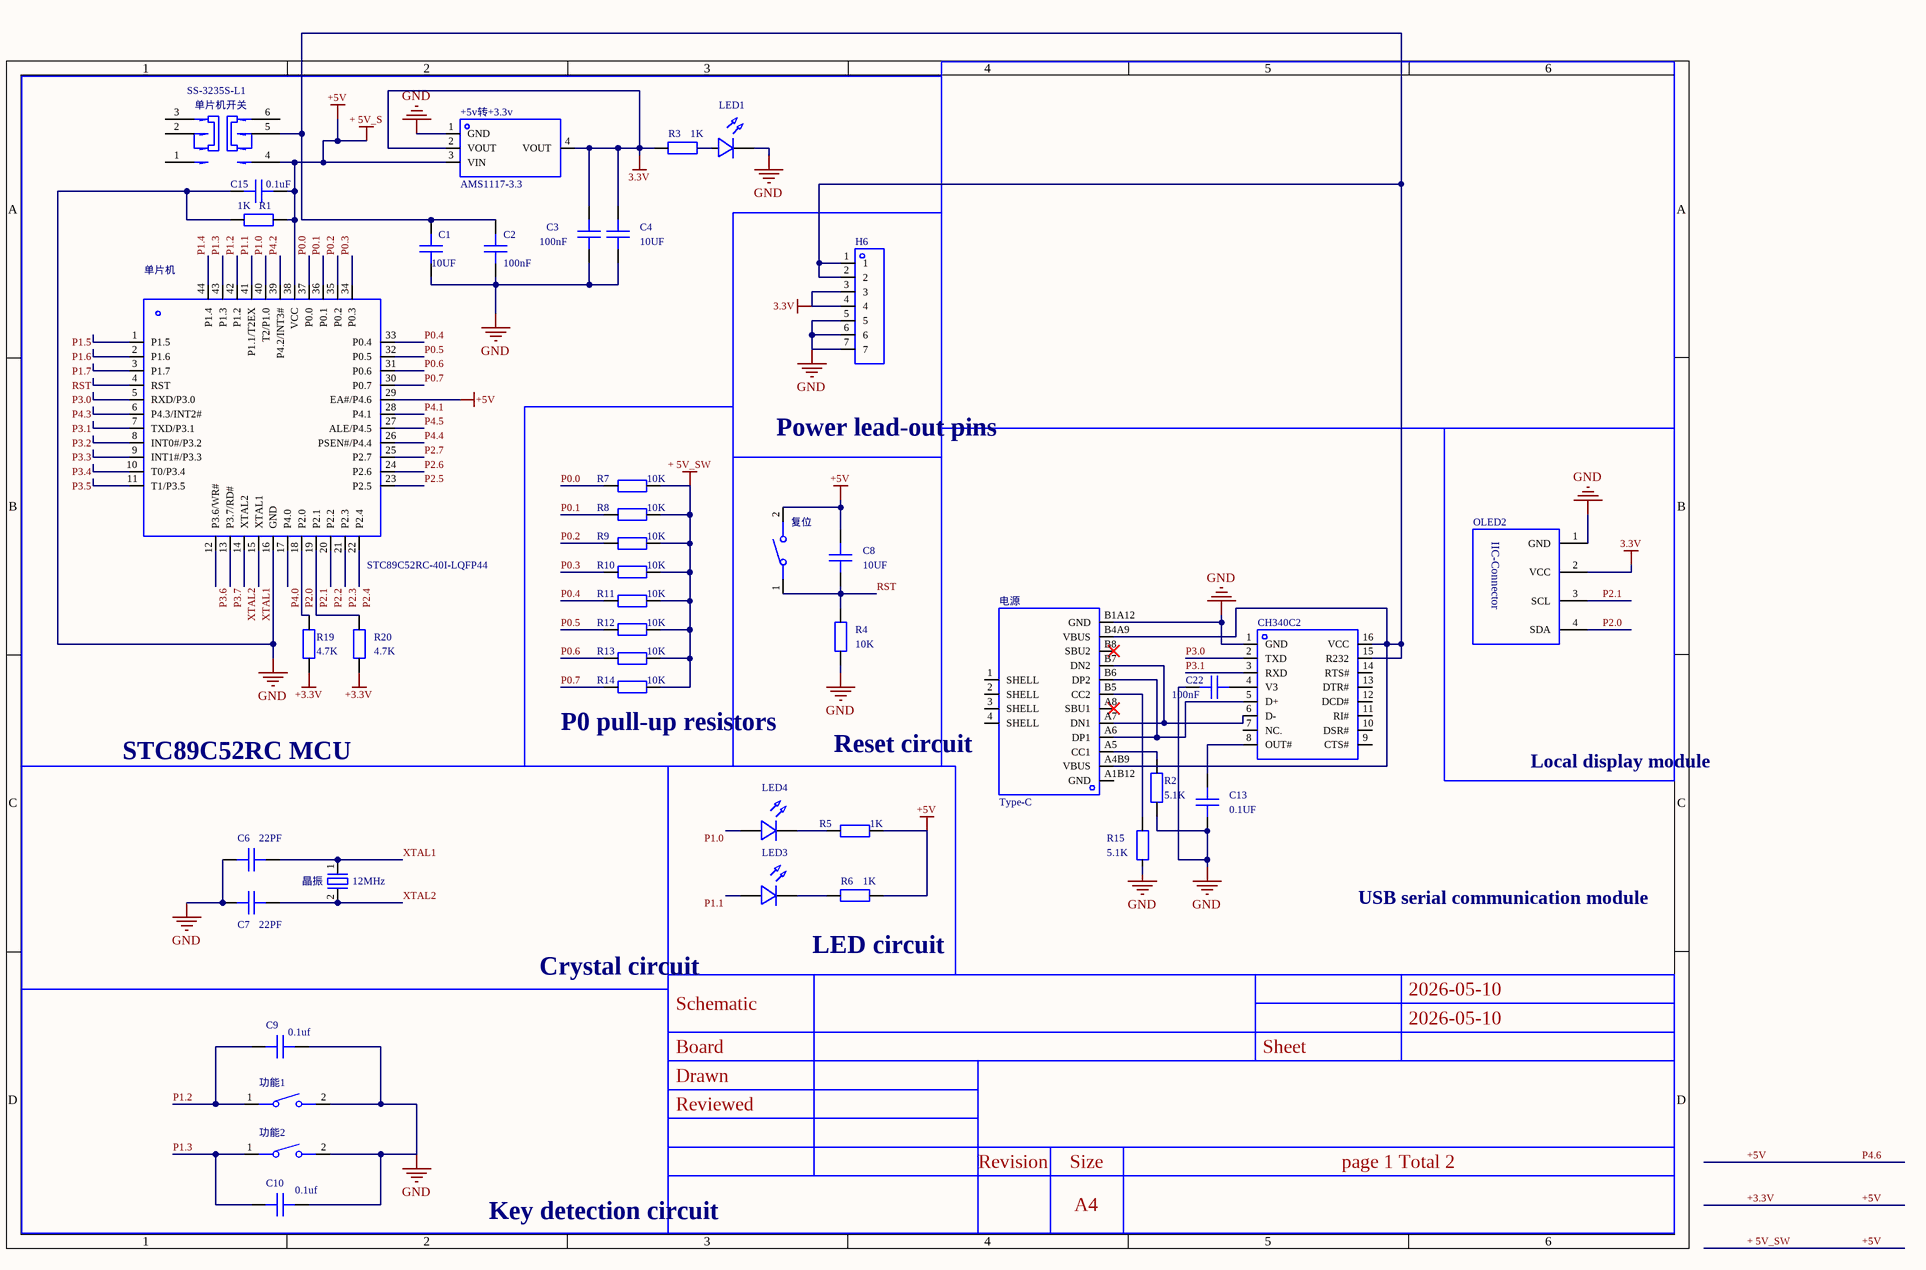
[diagram p0: MISC75115-3.schdoc]
# Altium project MISC75115-2.PrjPcb
2 sheets, 101 parts. Net scope: global (net labels, ports and power ports of the same name join across sheets).
Board file: MISC75115.pcbdoc
Sheets:
  MISC75115-3.schdoc
  MISC75115-4.schdoc

## Sheet MISC75115-3.schdoc
size 297 x 209 mm; Version: V1.0; @Project Name: MISC75115; @Page Count: 2; @Update Date: 2026-05-22; @Create Date: 2026-05-22; @Schematic Name: MISC75115; @Page No: 1; @Board Name: MISC75115; @Create Time: 00:24:12; @Update Time: 02:37:15; Size: A4

### Parts
+5v转+3.3v  AMS1117-3.3  [SOT-223-3_L6.5-W3.4-P2.30-LS7.0-BR]
C1  10UF  [C0805]
C2  100nF  [C0805]
C3  100nF  [C0805]
C4  10UF  [C0805]
C6  22PF  [C0805]
C7  22PF  [C0805]
C8  10UF  [C0805]
C9  0.1uf  [C0805]
C10  0.1uf  [C0805]
C13  0.1UF  [C0805]
C15  0.1uF  [C0805]
C22  100nF  [C0603]
CH340C2  CH340C  [SOP-16_L10.0-W3.9-P1.27-LS6.0-BL]  (value not drawn)
H6  (no value)  [HDR-TH_7P-P2.54-V-M]
LED1  (no value)  [LED_0805]
LED3  (no value)  [LED_0805]
LED4  (no value)  [LED_0805]
OLED2  0.96OLED_4P_MODULE_JX  [0.96OLED_4P]  (value not drawn)
R1  1K  [R0805]
R2  5.1K  [R0603]
R3  1K  [R0805]
R4  10K  [R0805]
R5  1K  [R0805]
R6  1K  [R0805]
R7  10K  [R0805]
R8  10K  [R0805]
R9  10K  [R0805]
R10  10K  [R0805]
R11  10K  [R0805]
R12  10K  [R0805]
R13  10K  [R0805]
R14  10K  [R0805]
R15  5.1K  [R0603]
R19  4.7K  [R0603]
R20  4.7K  [R0603]
功能1  Tact switch 3*4*H  [SW-SMD_L4.0-W2.9-LS5.0]  (value not drawn)
功能2  Tact switch 3*4*H  [SW-SMD_L4.0-W2.9-LS5.0]  (value not drawn)
单片机  STC89C52RC-40I-LQFP44  [LQFP-44_L10.0-W10.0-P0.80-LS12.0-BL]
单片机开关  SS-3235S-L1  [SW-SMD_SS-3235S-LX]
复位  Tact switch 3*4*H  [SW-SMD_L4.0-W2.9-LS5.0]  (value not drawn)
晶振  12MHz  [CRYSTAL-SMD_L11.4-W4.7-LS12.7]
电源  Type-C  [USB-C-SMD_TYPE-C16PIN]

### Blocks framed on the sheet
STC89C52RC MCU: +5v转+3.3v C1-C4 C15 LED1 R1 R3 R19 R20 单片机 单片机开关
Power lead-out pins: H6
P0 pull-up resistors: R7-R14
Reset circuit: C8 R4 复位
Local display module: OLED2

### Nets
3.3V: +5v转+3.3v.2(VOUT) +5v转+3.3v.4(VOUT) C3.2 C4.2 H6.3 H6.4 OLED2.2(VCC) R3.1
+ 5V_SW: +5v转+3.3v.3(VIN) C8.1 C15.2 R1.2 R5.2 R6.2 R7.2 R8.2 R9.2 R10.2 R11.2 R12.2 R13.2 R14.2 R19.1 R20.1 单片机.29(EA#/P4.6) 单片机.38(VCC) 单片机开关.4 复位.2  [also labelled + 5V_S, +3.3V, +5V, P4.6]
GND: +5v转+3.3v.1(GND) C1.1 C2.1 C3.1 C4.1 C6.2 C7.2 C9.1 C10.1 C13.1 C15.1 C22.1 CH340C2.1(GND) H6.5 H6.6 H6.7 LED1.1(C) OLED2.1(GND) R1.1 R2.1 R4.1 R15.1 功能1.2 功能2.2 单片机.16(GND) 电源.B1A12(GND)
P0.0: R7.1 单片机.37(P0.0)
P0.1: R8.1 单片机.36(P0.1)
P0.2: R9.1 单片机.35(P0.2)
P0.3: R10.1 单片机.34(P0.3)
P0.4: R11.1 单片机.33(P0.4)
P0.5: R12.1 单片机.32(P0.5)
P0.6: R13.1 单片机.31(P0.6)
P0.7: R14.1 单片机.30(P0.7)
P1.0: LED4.2(A) 单片机.40(T2/P1.0)
P1.1: LED3.2(A) 单片机.41(P1.1/T2EX)
P1.2: C9.2 功能1.1 单片机.42(P1.2)
P1.3: C10.2 功能2.1 单片机.43(P1.3)
P1.4: 单片机.44(P1.4)
P1.5: 单片机.1(P1.5)
P1.6: 单片机.2(P1.6)
P1.7: 单片机.3(P1.7)
P2.0: OLED2.4(SDA) R19.2 单片机.18(P2.0)
P2.1: OLED2.3(SCL) R20.2 单片机.19(P2.1)
P2.2: 单片机.20(P2.2)
P2.3: 单片机.21(P2.3)
P2.4: 单片机.22(P2.4)
P2.5: 单片机.23(P2.5)
P2.6: 单片机.24(P2.6)
P2.7: 单片机.25(P2.7)
P3.0: CH340C2.2(TXD) 单片机.5(RXD/P3.0)
P3.1: CH340C2.3(RXD) 单片机.7(TXD/P3.1)
P3.2: 单片机.8(INT0#/P3.2)
P3.3: 单片机.9(INT1#/P3.3)
P3.4: 单片机.10(T0/P3.4)
P3.5: 单片机.11(T1/P3.5)
P3.6: 单片机.12(P3.6/WR#)
P3.7: 单片机.13(P3.7/RD#)
P4.0: 单片机.17(P4.0)
P4.1: 单片机.28(P4.1)
P4.2: 单片机.39(P4.2/INT3#)
P4.3: 单片机.6(P4.3/INT2#)
P4.4: 单片机.26(PSEN#/P4.4)
P4.5: 单片机.27(ALE/P4.5)
RST: C8.2 R4.2 单片机.4(RST) 复位.1
XTAL1: C6.1 单片机.15(XTAL1) 晶振.1
XTAL2: C7.1 单片机.14(XTAL2) 晶振.2(GND)
NetC1_2: C1.2 C2.2 CH340C2.15(R232) CH340C2.16(VCC) H6.1 H6.2 单片机开关.5 电源.A4B9(VBUS) 电源.B4A9(VBUS)
NetC13_2: C13.2 CH340C2.8(OUT#)
NetC22_2: C22.2 CH340C2.4(V3)
NetCH340C2_5: CH340C2.5(D+) 电源.A6(DP1) 电源.B6(DP2)
NetCH340C2_6: CH340C2.6(D-) 电源.A7(DN1) 电源.B7(DN2)
NetLED1_2: LED1.2(A) R3.2
NetLED3_1: LED3.1(C) R6.1
NetLED4_1: LED4.1(C) R5.1
NetR2_2: R2.2 电源.A5(CC1)
NetR15_2: R15.2 电源.B5(CC2)

Not connected (* = marked no-connect by the designer): CH340C2 7(NC.) 9(CTS#) 10(DSR#) 11(RI#) 12(DCD#) 13(DTR#) 14(RTS#); 单片机开关 1 2 3 6; 电源 1(SHELL) 2(SHELL) 3(SHELL) 4(SHELL) A1B12(GND) A8(SBU1)* B8(SBU2)*

### Notes on the sheet
- USB serial communication module
- Crystal circuit
- LED circuit
- Key detection circuit
- 2026-05-10
- Schematic
- Board
- Sheet
- Drawn
- Reviewed
- Revision
- Size
- A4
- page 1 Total 2

### Library data of the parts
+5v转+3.3v = AMS1117-3.3_C6186: Output type: fixed; working voltage: 15V; output voltage: 3.3V; output current: 1A; PSRR: 72dB@(120Hz); output polarity: positive;; Manufacturer: AMS; AddInBom: yes; Voltage Dropout: 1.1V@(800mA); standby current: 5mA; Noise: 0.003%Vout; Number of Outputs: 1; ModelId: 925194bf9823436183a3e0b978a8d076; ModelName: SOT-223-4P_L6.5-W3.5-H1.6-LS7.0-P2.30; ModelTransform: 279.89794,255.905,0,180,0,0,-3.9385,-0.0005,0; Device: AMS1117-3.3_C6186; Symbol: AMS1117-3.3; FootprintName: SOT-223-3_L6.5-W3.4-P2.30-LS7.0-BR; LCSC Part Name: 3.3V 1A 15V; SupplierPart: C6186; ManufacturerPart: AMS1117-3.3; Supplier Footprint: SOT-223; JLCPCB Part Class: JLCPCB Part Class  Basic library; Datasheet: https://item.szlcsc.com/datasheet/AMS1117-3.3/6652.html; Supplier: LCSC; ConvertToPcb: yes; Output Type: Fixed; Voltage - Supply: 15V; Output Voltage: 3.3V; Output Current: 1A; Power Supply Rejection Ratio (PSRR): 72dB@(120Hz); Features: Overcurrent protection; thermal shutdown; Operating Temperature: -40℃~+125℃; Output Configuration: Positive
C1-C4 C8 = CAP_0805: Symbol: Capacitance; ConvertToPcb: yes; ModelId: 1ba041120af144c991958decab20d241; ModelName: C0805_L2.0-W1.3-H1.3; ModelTransform: 78.74,51.181,0,0,0,0,0,0.0005,0; Device: CAP_0805; FootprintName: C0805; AddInBom: yes; Supplier Footprint: 0805
  C1 C4 C8: Value: 10UF
  C2 C3: Value: 100nF
C6 C7 C9 C10 = CAP_0805: SymbolName: Capacitance; ConvertToPcb: yes; ModelId: 1ba041120af144c991958decab20d241; ModelName: C0805_L2.0-W1.3-H1.3; ModelTransform: 78.74,51.181,0,0,0,0,0,0.0005,0; Device: CAP_0805; FootprintName: C0805; AddInBom: yes; Supplier Footprint: 0805
  C6 C7: Value: 22PF
  C9 C10: Value: 0.1uf
C13 C15 = CAP_0805: Symbol: Capacitance; 3D Model: 1ba041120af144c991958decab20d241; 3D Model Transform: 78.74,51.181,0,0,0,0,0,0.0005,0; ConvertToPcb: yes; ModelName: C0805_L2.0-W1.3-H1.3; Device: CAP_0805; Supplier Footprint: 0805; FootprintName: C0805; AddInBom: yes
  C13: Value: 0.1UF
  C15: Value: 0.1uF
C22 = CAP_0603: Symbol: Capacitance; 3D Model: ac125912035d415993ca9572d50418b1; 3D Model Transform: 62.992,31.496,0,0,0,0,0,0,0; ConvertToPcb: yes; ModelName: C0603_L1.6-W0.8-H0.8; Device: CAP_0603; Supplier Footprint: 0603; Value: 100nF; FootprintName: C0603; AddInBom: yes
CH340C2 = CH340C: Application function: transceiver; USB protocol version: USB 2.0; data rate: 2Mbps;; Manufacturer: WCH(南京沁恒); 3D Model: 3361a6792abf4a8f8fbca4f1924a67ee; 3D Model Transform: 240.39054,393.7,0,90,0,0,0,0,0; USB Protocol: USB 2.0; Voltage - Supply: 3.3V; 5V; Current - Supply: 7mA; Supply Current (Iq): 50uA; AddInBom: yes; ModelName: SOP-16_L9.9-W3.9-H1.5-LS6.0-P1.27; Device: CH340C; Symbol: CH340C; LCSC Part Name: USB转串口芯片; Supplier Part: C84681; Manufacturer Part: CH340C; Supplier Footprint: SOP-16; JLCPCB Part Class: JLCPCB Part Class  Extended library; Datasheet: https://item.szlcsc.com/datasheet/CH340C/85852.html; Supplier: LCSC; Applications Function: Transceiver; Data Rate: 2Mbps; Operating Temperature: -20℃~+70℃; FootprintName: SOP-16_L10.0-W3.9-P1.27-LS6.0-BL; ConvertToPcb: yes
H6 = HDR-M_2.54_1x7P: Symbol: PZ254V-11-07P; ConvertToPcb: yes; ModelId: 3f496cdc752348c6a5e9157bbaceaf96; ModelName: HDR-TH_7P-P2.54-M-LI-1X7P; ModelTransform: 690.1561,98.425,0,0,0,0,0,0,-118.11; Device: HDR-M_2.54_1x7P; FootprintName: HDR-TH_7P-P2.54-V-M; AddInBom: yes; SupplierPart: C492406; Supplier Footprint: 插件
LED1 LED3 LED4 = LED_0805-G: Symbol: LED_G; Convert to PCB: yes; 3D Model: 381ae4d721d6485eaad9d0ca067812b5; 3D Model Transform: 63.9,39.8,31.9,0,0,0,0,0,0; ModelName: LED-0805_G; Device: LED_0805-G; Add into BOM: yes; Supplier Footprint: 0805; FootprintName: LED_0805
OLED2 = 0.96OLED_4P_MODULE_JX: 3D Model: 79c000fdb68d45a296c2e9bedf4f9055; 3D Model Transform: 1393.69792,1318.895,0,0,0,0,0,-560.079,-137.795; AddInBom: yes; Device: 0.96OLED_4P_MODULE_JX; Symbol: 0.96OLED_4P_MODULE_JX; LCSC Part Name: 0.96OLED_4P_MODULE_JX; Supplier Part: C9900004566; Manufacturer Part: 0.96OLED_4P_MODULE_JX; Supplier Footprint: 插件; JLCPCB Part Class: JLCPCB Part Class  Extended library; Supplier: LCSC; FootprintName: 0.96OLED_4P; ConvertToPcb: yes; ModelName: 0.96OLED_4P
R1 = Res_0805: Symbol: Resistor; 3D Model: 37a81e68749a4138bd2dfa6897b24b85; 3D Model Transform: 78.74,51.181,0,0,0,0,0,-0.0005,0; ConvertToPcb: yes; ModelName: R0805_L2.0-W1.3-H0.6; Device: Res_0805; Supplier Footprint: 0805; Value: 1K; FootprintName: R0805; AddInBom: yes
R2 R15 = Res_0603: Symbol: Resistor; 3D Model: fc143cca1e79419f9cd78b61e9279f08; 3D Model Transform: 31.8897,63.7794,0,90,0,0,0,0,0; ConvertToPcb: yes; Device: Res_0603; Value: 5.1K; Supplier Footprint: 0603; FootprintName: R0603; AddInBom: yes; ModelName: R0603
R3 R4 R7-R14 = Res_0805: Symbol: Resistor; ConvertToPcb: yes; ModelId: 349bb002ce6c6897; ModelName: R0805_L2.0-W1.3-H0.6; ModelTransform: 0,0,0,0,0,0,0,0,0; Device: Res_0805; FootprintName: R0805; AddInBom: yes; Supplier Footprint: 0805
  R3: Value: 1K
  R4 R7-R14: Value: 10K
R5 R6 = Res_0805: SymbolName: Resistor; ConvertToPcb: yes; ModelId: 349bb002ce6c6897; ModelName: R0805_L2.0-W1.3-H0.6; ModelTransform: 0,0,0,0,0,0,0,0,0; Device: Res_0805; Value: 1K; FootprintName: R0805; AddInBom: yes; Supplier Footprint: 0805
R19 R20 = Res_0603: Symbol: Resistor; ConvertToPcb: yes; ModelId: c5da5eb17d71f24d; ModelTransform: 0,0,0,0,0,0,0,0,0; Device: Res_0603; Value: 4.7K; FootprintName: R0603; AddInBom: yes; Supplier Footprint: 0603; ModelName: R0603
功能1 功能2 复位 = 轻触按键3*4*H: AddInBom: yes; ModelId: 63599cce708d48afbce1b0db00354477; ModelName: SW-SMD_L4.0-W2.9-H2-LS5.0; ModelTransform: 196.85,114.173,0,0,0,0,0,0,0; Device: Tact switch 3*4*H; Symbol: Tact switch 3*4*H; FootprintName: SW-SMD_L4.0-W2.9-LS5.0; LCSC Part Name: 轻触按键3*4*H; SupplierPart: C9900017573; ManufacturerPart: 轻触按键3*4*H; Supplier Footprint: 轻触按键3*4*2.5; JLCPCB Part Class: JLCPCB Part Class  Extended library; Supplier: LCSC; ConvertToPcb: yes
单片机 = STC89C52RC-40I-LQFP44: CPU core: 51 family;; Manufacturer: STC; Symbol: STC89C52RC-40I_C8707; AddInBom: yes; Program Storage Size: 8KB; Program Memory Type: FLASH; Number of I/O: 39; Voltage - Supply: 3.3V~5.5V; ModelId: cfc67ede9fd147078f17820e55193bca; ModelName: LQFP-44_L10.0-W10.0-H1.4-LS12.0-P0.80; ModelTransform: 472.441,472.441,0,0,0,0,0,0,0; Device: STC89C52RC-40I-LQFP44; FootprintName: LQFP-44_L10.0-W10.0-P0.80-LS12.0-BL; LCSC Part Name: 单片机原理及应用; SupplierPart: C8707; ManufacturerPart: STC89C52RC-40I-LQFP44; Supplier Footprint: LQFP-44(10x10); JLCPCB Part Class: JLCPCB Part Class  Extended library; Datasheet: https://item.szlcsc.com/datasheet/STC89C52RC-40I-LQFP44/9213.html; Supplier: LCSC; ConvertToPcb: yes; CPU Core: 51 family
单片机开关 = SS-3235S-L1: Circuit: DPDT; mounting: flat mount; switch colour: black; rated current: 50mA; rated voltage: 12V; service life: 1万 cycles;; Manufacturer: XKB Connection(中国星坤); AddInBom: yes; Actuator Style: Rectangular column; Switch Height: 3.2mm; ModelId: 81e407adedd8b3e1; ModelTransform: 0,0,0,0,0,0,0,0,0; Device: SS-3235S-L1; Symbol: SS-3235S-L1; FootprintName: SW-SMD_SS-3235S-LX; LCSC Part Name: 柄长2mm 卧贴双档 滑动开关; SupplierPart: C500055; ManufacturerPart: SS-3235S-L1; Supplier Footprint: SMD,9.1x3.6mm; JLCPCB Part Class: JLCPCB Part Class  Extended library; Datasheet: https://item.szlcsc.com/datasheet/SS-3235S-L1/512181.html; Supplier: LCSC; ConvertToPcb: yes; Termination Style: Gull-wing; Length: 9.1mm; Width: 3.55mm; Mounting Type: Flat mount; Actuator Color: Black; Current Rating: 50mA; Voltage Rating: 12V; Life: 1万 cycles; Operating Temperature: -40℃~+85℃; ModelName: SW-SMD_SS-3235S-LX
晶振 = ABLS-12.000MHZ-B4H-T: Frequency: 12MHz; frequency tolerance at room temperature: ±30ppm; load capacitance: 18pF; frequency stability: ±35ppm;; Manufacturer: ABRACON; AddInBom: yes; Equivalent Series Resistance(ESR): 50Ω; ModelId: be19d32e6d024fb4863eb8f4e3f5efcc; ModelTransform: 499.999,185.039,0,0,0,0,0,0,0; Device: ABLS-12.000MHZ-B4H-T; Symbol: ABLS-12.000MHZ-B4H-T; FootprintName: CRYSTAL-SMD_L11.4-W4.7-LS12.7; LCSC Part Name: 12MHz ±30ppm 18pF; SupplierPart: C1986452; ManufacturerPart: ABLS-12.000MHZ-B4H-T; Supplier Footprint: HC-49S-SMD; JLCPCB Part Class: JLCPCB Part Class  Extended library; Datasheet: https://item.szlcsc.com/datasheet/ABLS-12.000MHZ-B4H-T/2077997.html; Supplier: LCSC; ConvertToPcb: yes; Value: 12MHz; Normal temperature Frequency Tolerance: ±30ppm; Load Capacitance: 18pF; Frequency Stability: ±35ppm; Operating Temperature: -20℃~+70℃; ModelName: CRYSTAL-SMD_L11.4-W4.7-LS12.7
电源 = Type-C-TOP_1: 3D Model: d6783d3a2268456b863f42d3286191d0; 3D Model Transform: 351.9678,311.023,0,180,0,0,0,-41.85,-39.37; AddInBom: yes; Device: Type-C-TOP_1; Symbol: TYPE-C-TOP_1; LCSC Part Name: Type-C-TOP_1; Supplier Part: C9900005857; Manufacturer Part: Type-C; Supplier Footprint: Type-C16P; JLCPCB Part Class: JLCPCB Part Class  Extended library; Supplier: LCSC; FootprintName: USB-C-SMD_TYPE-C16PIN; ConvertToPcb: yes; ModelName: USB-C-SMD_TYPE-C16PIN

## Sheet MISC75115-4.schdoc
size 297 x 209 mm; Version: V1.0; @Project Name: MISC75115; @Page Count: 1; @Update Date: 2026-05-22; @Create Date: 2026-05-22; @Schematic Name: MISC75115; @Page No: 0; @Board Name: MISC75115; @Create Time: 05:59:13; @Update Time: 05:59:13; Size: A4
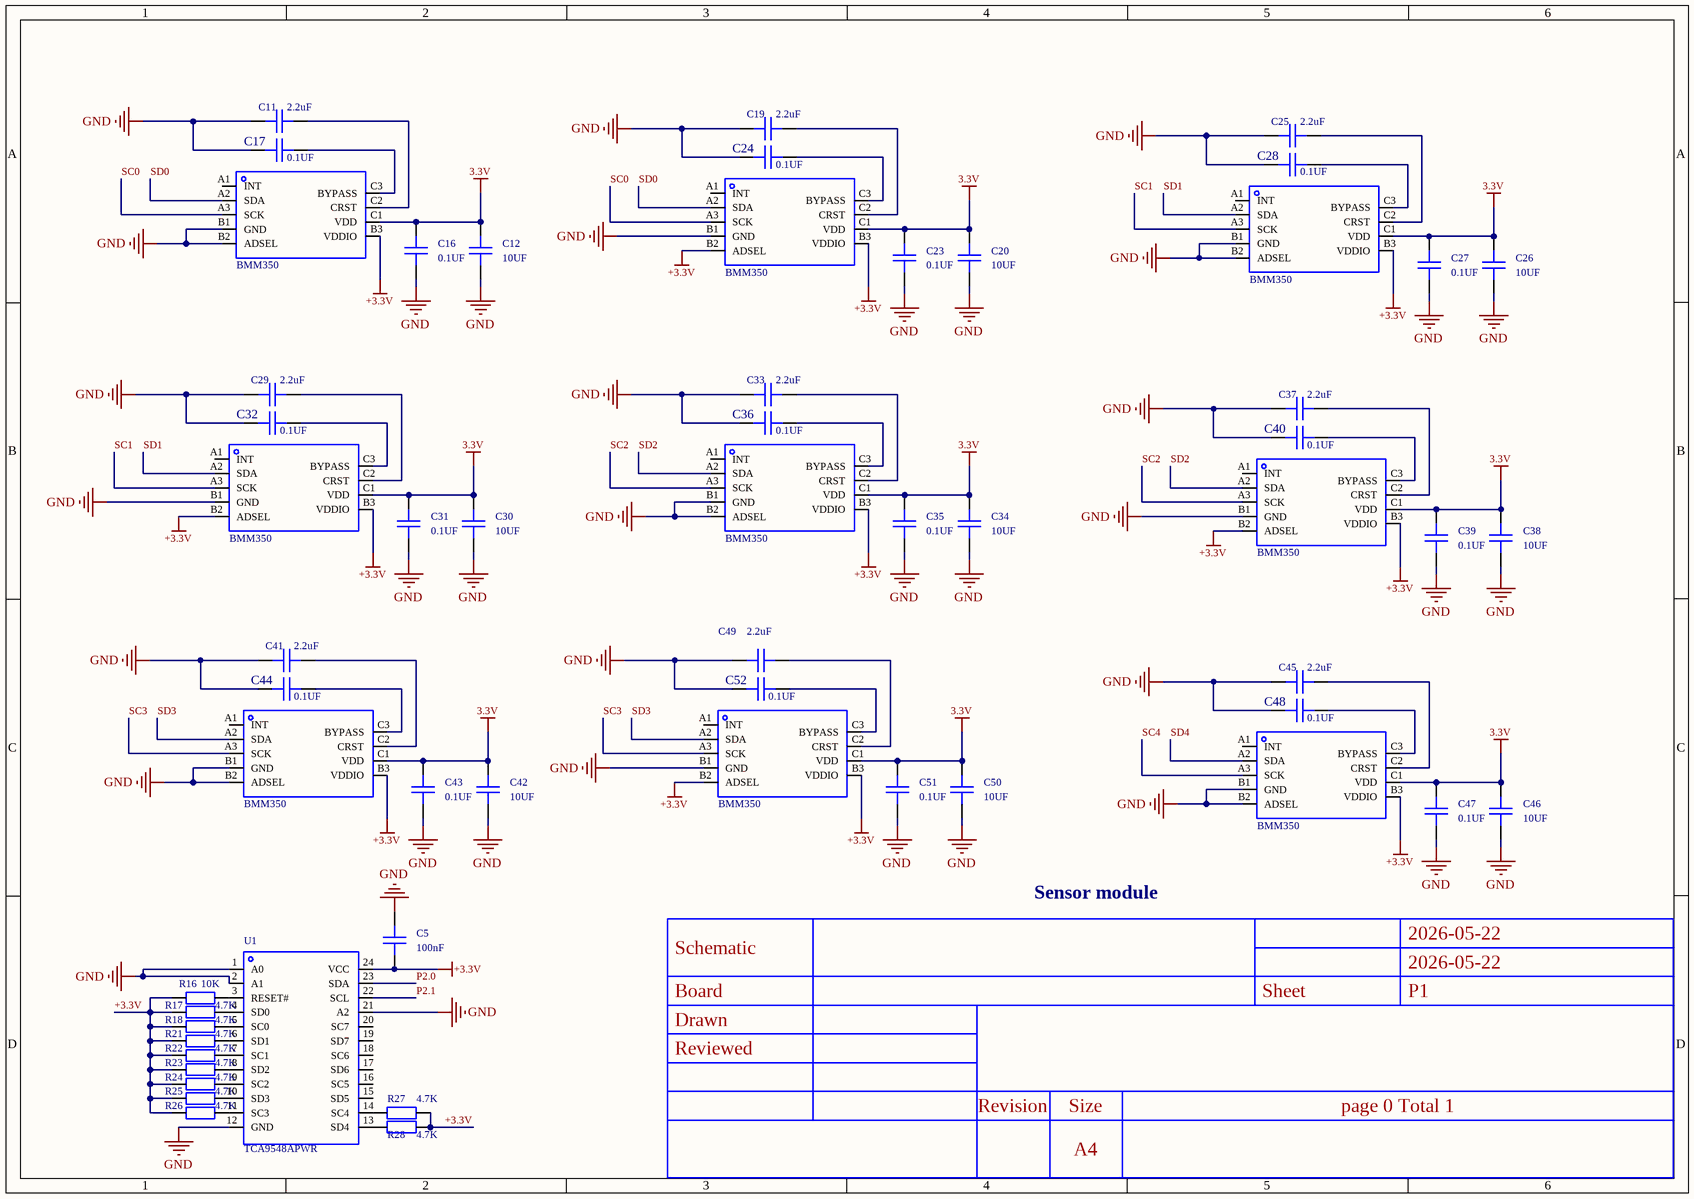
[diagram p1: MISC75115-4.schdoc]

### Parts
C5  100nF  [C0805]
C11  2.2uF  [C0805]
C12  10UF  [C0805]
C16  0.1UF  [C0805]
C17  0.1UF  [C0805]
C19  2.2uF  [C0805]
C20  10UF  [C0805]
C23  0.1UF  [C0805]
C24  0.1UF  [C0805]
C25  2.2uF  [C0805]
C26  10UF  [C0805]
C27  0.1UF  [C0805]
C28  0.1UF  [C0805]
C29  2.2uF  [C0805]
C30  10UF  [C0805]
C31  0.1UF  [C0805]
C32  0.1UF  [C0805]
C33  2.2uF  [C0805]
C34  10UF  [C0805]
C35  0.1UF  [C0805]
C36  0.1UF  [C0805]
C37  2.2uF  [C0805]
C38  10UF  [C0805]
C39  0.1UF  [C0805]
C40  0.1UF  [C0805]
C41  2.2uF  [C0805]
C42  10UF  [C0805]
C43  0.1UF  [C0805]
C44  0.1UF  [C0805]
C45  2.2uF  [C0805]
C46  10UF  [C0805]
C47  0.1UF  [C0805]
C48  0.1UF  [C0805]
C49  2.2uF  [C0805]
C50  10UF  [C0805]
C51  0.1UF  [C0805]
C52  0.1UF  [C0805]
R16  10K  [R0805]
R17  4.7K  [R0805]
R18  4.7K  [R0805]
R21  4.7K  [R0805]
R22  4.7K  [R0805]
R23  4.7K  [R0805]
R24  4.7K  [R0805]
R25  4.7K  [R0805]
R26  4.7K  [R0805]
R27  4.7K  [R0805]
R28  4.7K  [R0805]
U1  TCA9548APWR  [TSSOP-24_L7.8-W4.4-P0.65-LS6.4-BL]
U2  BMM350  [WLCSP-9_L1.3-W1.3-R3-C3-P0.40-TL]
U3  BMM350  [WLCSP-9_L1.3-W1.3-R3-C3-P0.40-TL]
U4  BMM350  [WLCSP-9_L1.3-W1.3-R3-C3-P0.40-TL]
U5  BMM350  [WLCSP-9_L1.3-W1.3-R3-C3-P0.40-TL]
U6  BMM350  [WLCSP-9_L1.3-W1.3-R3-C3-P0.40-TL]
U7  BMM350  [WLCSP-9_L1.3-W1.3-R3-C3-P0.40-TL]
U8  BMM350  [WLCSP-9_L1.3-W1.3-R3-C3-P0.40-TL]
U9  BMM350  [WLCSP-9_L1.3-W1.3-R3-C3-P0.40-TL]
U10  BMM350  [WLCSP-9_L1.3-W1.3-R3-C3-P0.40-TL]

### Nets
3.3V: C12.1 C16.2 C20.1 C23.2 C26.1 C27.2 C30.1 C31.2 C34.1 C35.2 C38.1 C39.2 C42.1 C43.2 C46.1 C47.2 C50.1 C51.2 U2.C1(VDD) U3.C1(VDD) U4.C1(VDD) U5.C1(VDD) U6.C1(VDD) U7.C1(VDD) U8.C1(VDD) U9.C1(VDD) U10.C1(VDD)
+3.3V: C5.1 R16.1 R17.1 R18.1 R21.1 R22.1 R23.1 R24.1 R25.1 R26.1 R27.2 R28.2 U1.24(VCC) U2.B3(VDDIO) U3.B2(ADSEL) U3.B3(VDDIO) U4.B3(VDDIO) U5.B2(ADSEL) U5.B3(VDDIO) U6.B3(VDDIO) U7.B2(ADSEL) U7.B3(VDDIO) U8.B3(VDDIO) U9.B3(VDDIO) U10.B2(ADSEL) U10.B3(VDDIO)  [project net + 5V_SW]
GND: C5.2 C11.2 C12.2 C16.1 C17.1 C19.2 C20.2 C23.1 C24.1 C25.2 C26.2 C27.1 C28.1 C29.2 C30.2 C31.1 C32.1 C33.2 C34.2 C35.1 C36.1 C37.2 C38.2 C39.1 C40.1 C41.2 C42.2 C43.1 C44.1 C45.2 C46.2 C47.1 C48.1 C49.2 C50.2 C51.1 C52.1 U1.1(A0) U1.2(A1) U1.12(GND) U1.21(A2) U2.B1(GND) U2.B2(ADSEL) U3.B1(GND) U4.B1(GND) U4.B2(ADSEL) U5.B1(GND) U6.B1(GND) U6.B2(ADSEL) U7.B1(GND) U8.B1(GND) U8.B2(ADSEL) U9.B1(GND) U9.B2(ADSEL) U10.B1(GND)
P2.0: U1.23(SDA)
P2.1: U1.22(SCL)
SC0: U2.A3(SCK) U3.A3(SCK)
SC1: U4.A3(SCK) U5.A3(SCK)
SC2: U6.A3(SCK) U7.A3(SCK)
SC3: U8.A3(SCK) U10.A3(SCK)
SC4: U9.A3(SCK)
SD0: U2.A2(SDA) U3.A2(SDA)
SD1: U4.A2(SDA) U5.A2(SDA)
SD2: U6.A2(SDA) U7.A2(SDA)
SD3: U8.A2(SDA) U10.A2(SDA)
SD4: U9.A2(SDA)
NetC11_1: C11.1 U2.C2(CRST)
NetC17_2: C17.2 U2.C3(BYPASS)
NetC19_1: C19.1 U3.C2(CRST)
NetC24_2: C24.2 U3.C3(BYPASS)
NetC25_1: C25.1 U4.C2(CRST)
NetC28_2: C28.2 U4.C3(BYPASS)
NetC29_1: C29.1 U5.C2(CRST)
NetC32_2: C32.2 U5.C3(BYPASS)
NetC33_1: C33.1 U6.C2(CRST)
NetC36_2: C36.2 U6.C3(BYPASS)
NetC37_1: C37.1 U7.C2(CRST)
NetC40_2: C40.2 U7.C3(BYPASS)
NetC41_1: C41.1 U8.C2(CRST)
NetC44_2: C44.2 U8.C3(BYPASS)
NetC45_1: C45.1 U9.C2(CRST)
NetC48_2: C48.2 U9.C3(BYPASS)
NetC49_1: C49.1 U10.C2(CRST)
NetC52_2: C52.2 U10.C3(BYPASS)
NetR16_2: R16.2 U1.3(RESET#)
NetR17_2: R17.2 U1.4(SD0)
NetR18_2: R18.2 U1.5(SC0)
NetR21_2: R21.2 U1.6(SD1)
NetR22_2: R22.2 U1.7(SC1)
NetR23_2: R23.2 U1.8(SD2)
NetR24_2: R24.2 U1.9(SC2)
NetR25_2: R25.2 U1.10(SD3)
NetR26_2: R26.2 U1.11(SC3)
NetR27_1: R27.1 U1.14(SC4)
NetR28_1: R28.1 U1.13(SD4)

Not connected (* = marked no-connect by the designer): U1 15(SD5) 16(SC5) 17(SD6) 18(SC6) 19(SD7) 20(SC7); U2 A1(INT); U3 A1(INT); U4 A1(INT); U5 A1(INT); U6 A1(INT); U7 A1(INT); U8 A1(INT); U9 A1(INT); U10 A1(INT)

### Notes on the sheet
- Sensor module
- 2026-05-22
- Schematic
- Board
- Sheet
- P1
- Drawn
- Reviewed
- Revision
- Size
- A4
- page 0 Total 1

### Library data of the parts
C5 = CAP_0805: Symbol: Capacitance; 3D Model: 1ba041120af144c991958decab20d2410819f05c4eef4c71ace90d822a990e87; 3D Model Transform: 78.74,51.181,0,0,0,0,0,0.0005,0; ConvertToPcb: yes; ModelName: C0805_L2.0-W1.3-H1.3; Device: CAP_0805; Supplier Footprint: 0805; Value: 100nF; AddInBom: yes; FootprintName: C0805
C11 C19 C25 C29 C33 C37 C41 C45 C49 = CGB4B3X7R0J225K055AB: Capacitance: 2.2uF; tolerance: ±10%; rated voltage: 6.3V; dielectric (temperature coefficient): X7R;; Manufacturer: TDK; 3D Model: 1ba041120af144c991958decab20d2410819f05c4eef4c71ace90d822a990e87; 3D Model Transform: 78.74,51.181,0,0,0,0,0,0.0005,0; AddInBom: yes; ModelName: C0805_L2.0-W1.3-H1.3; Symbol: CGB4B3X7R0J225K055AB; Device: CGB4B3X7R0J225K055AB; LCSC Part Name: 2.2uF ±10% 6.3V; Supplier Part: C2179322; Manufacturer Part: CGB4B3X7R0J225K055AB; Supplier Footprint: 0805; JLCPCB Part Class: Extended Part; Datasheet: https://atta.szlcsc.com/upload/public/pdf/source/20191105/C343012_3F47E91403558E3EBEE82CA44A798D40.pdf; Supplier: LCSC; Value: 2.2uF; Tolerance: ±10%; Voltage Rated: 6.3V; Temperature Coefficient: X7R; FootprintName: C0805; ConvertToPcb: yes
C12 C16 C17 C20 C23 C24 C26-C28 C30-C32 C34-C36 C38-C40 C42-C44 C46-C48 C50-C52 = CAP_0805: as C13 on sheet MISC75115-3; Device: CAP_0805; Supplier Footprint: 0805; FootprintName: C0805; AddInBom: yes
  C12 C20 C26 C30 C34 C38 C42 C46 C50: Value: 10UF
  C16 C17 C23 C24 C27 C28 C31 C32 C35 C36 C39 C40 C43 C44 C47 C48 C51 C52: Value: 0.1UF
R16-R18 R21-R28 = Res_0805: Symbol: Resistor; 3D Model: 37a81e68749a4138bd2dfa6897b24b850819f05c4eef4c71ace90d822a990e87; 3D Model Transform: 78.74,51.181,0,0,0,0,0,-0.0005,0; ConvertToPcb: yes; ModelName: R0805_L2.0-W1.3-H0.6; Device: Res_0805; Supplier Footprint: 0805; AddInBom: yes; FootprintName: R0805
  R16: Value: 10K
  R17 R18 R21-R28: Value: 4.7K
U1 = TCA9548APWR: TCA9548A 8-channel, 1.65V to 5.5V I2C/SMBus switch with reset and voltage translation; Manufacturer: TI(德州仪器); AddInBom: yes; ModelId: 57e278220af748a2882c4abba4094eb90819f05c4eef4c71ace90d822a990e87; ModelName: TSSOP-24_L7.8-W4.4-H1.0-LS6.4-P0.65; ModelTransform: 252.188,307.086,0,90,0,0,0,0,0; Symbol: TCA9548APWR; Device: TCA9548APWR; LCSC Part Name: 支持复位的低压8通道I²C开关; SupplierPart: C130026; ManufacturerPart: TCA9548APWR; Supplier Footprint: TSSOP-24; JLCPCB Part Class: Extended Part; Datasheet: https://www.ti.com/cn/lit/gpn/tca9548a; Supplier: LCSC; ConvertToPcb: yes; FootprintName: TSSOP-24_L7.8-W4.4-P0.65-LS6.4-BL
U2-U10 = BMM350: 3D Model: 5e906eb31187499fa9dbe78db1290694; 3D Model Transform: 51.5747,51.181,0,0,0,0,0,0,0; AddInBom: yes; Symbol: BMM350; Device: BMM350; LCSC Part Name: BMM350; Supplier Part: C7496950; Manufacturer Part: BMM350; Supplier Footprint: BGA-9_1.28X1.28mm; JLCPCB Part Class: JLCPCB Part Class  Extended library; Supplier: LCSC; FootprintName: WLCSP-9_L1.3-W1.3-R3-C3-P0.40-TL; ConvertToPcb: yes; ModelName: WLCSP-9_L1.3-W1.3-R3-C3-P0.40-TL

## Nets that join several sheets
3.3V: MISC75115-3 (8 pins), MISC75115-4 (27 pins)
+ 5V_SW: MISC75115-3 (20 pins), MISC75115-4 (26 pins)
GND: MISC75115-3 (26 pins), MISC75115-4 (55 pins)
P2.0: MISC75115-3 (OLED2.4 R19.2 单片机.18), MISC75115-4 (U1.23)
P2.1: MISC75115-3 (OLED2.3 R20.2 单片机.19), MISC75115-4 (U1.22)